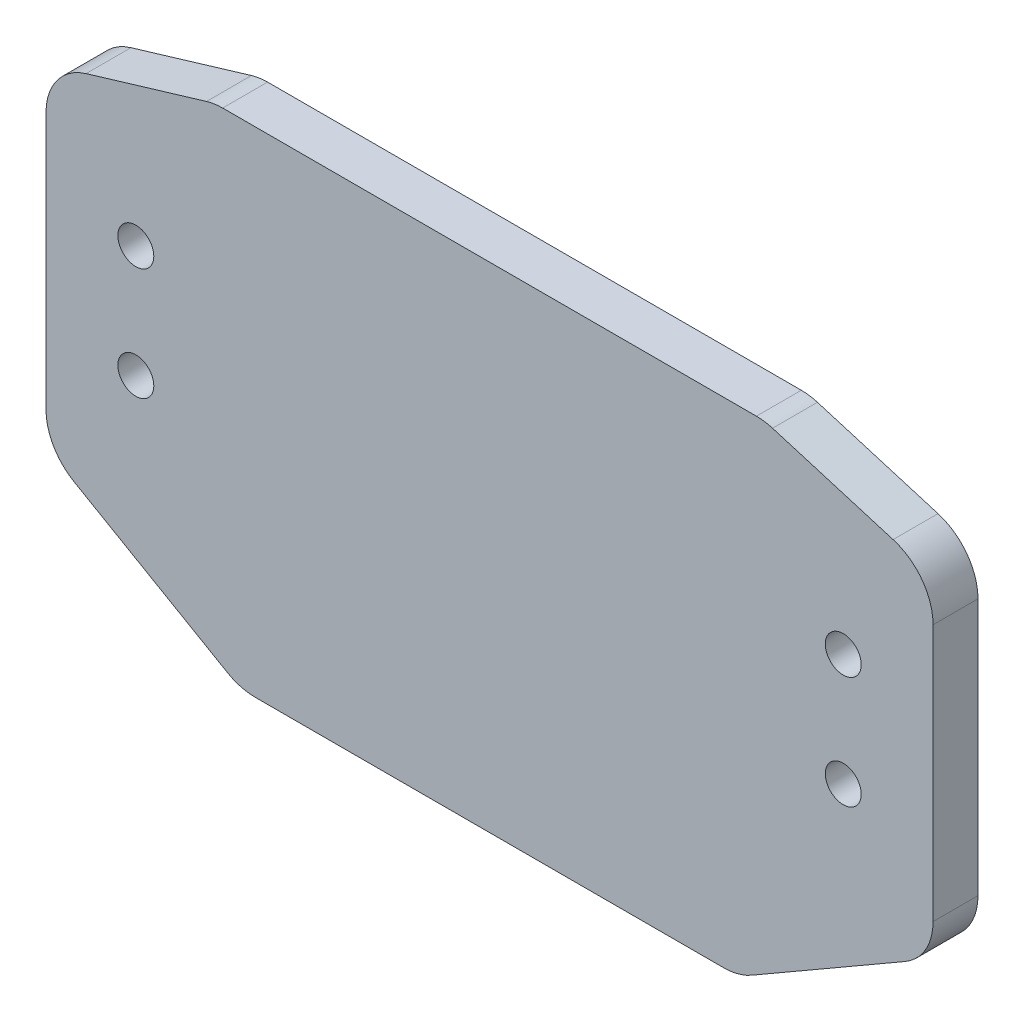
SolidWorks part; units mm, degrees
material "ABS PC"
ref_plane "前视基准面" through (0, 0, 0) normal (0, 0, 1) x (1, 0, 0)
ref_plane "上视基准面" through (0, 0, 0) normal (0, 1, 0) x (1, 0, 0)
ref_plane "右视基准面" through (0, 0, 0) normal (1, 0, 0) x (0, 0, -1)
sketch "草图1" plane through (0, 0, 0) normal (0, 0, 1) x (1, 0, 0)
  line L0 (0, 23.5) -> (0, -20.5) construction
  line L1 (-24.5, 23.5) -> (24.5, 23.5)
  line L2 (-39.5, 19) -> (-39.5, -10.5)
  line L3 (-22.1795, -20.5) -> (22.1795, -20.5)
  line L4 (39.5, 19) -> (39.5, -10.5)
  line L5 (-39.5, -10.5) -> (-22.1795, -20.5)
  line L6 (-39.5, 19) -> (-24.5, 23.5)
  line L7 (-31.5, 9) -> (-31.5, -1) construction
  line L8 (31.5, 9) -> (31.5, -1) construction
  line L9 (39.5, -10.5) -> (22.1795, -20.5)
  line L10 (39.5, 19) -> (24.5, 23.5)
  circle A0 centre (-31.5, 9) radius 1.6
  circle A1 centre (-31.5, -1) radius 1.6
  circle A2 centre (31.5, -1) radius 1.6
  circle A3 centre (31.5, 9) radius 1.6
  circle A4 centre (0, 0) radius 19.5 construction
  point P0 (0, 0)
  dimension "D1" = 79
  dimension "D4" = 3.2
  dimension "D7" = 39
  dimension "D2" = 10
  dimension "D3" = 8
  dimension "D5" = 1
  dimension "D6" = 44
  dimension "D8" = 14.5
  dimension "D9" = 10
  dimension "D10" = 49
  dimension "D11" = 120
  dimension "D12" = 10
extrude "凸台-拉伸1" add sketch "草图1" along normal blind 4
fillet "R5 圆角1" radius 5 8 edges at (-39.5, -10.5, 2) (-22.1795, -20.5, 2) (22.1795, -20.5, 2) (39.5, -10.5, 2) (39.5, 19, 2) (24.5, 23.5, 2) (-24.5, 23.5, 2) (-39.5, 19, 2)
